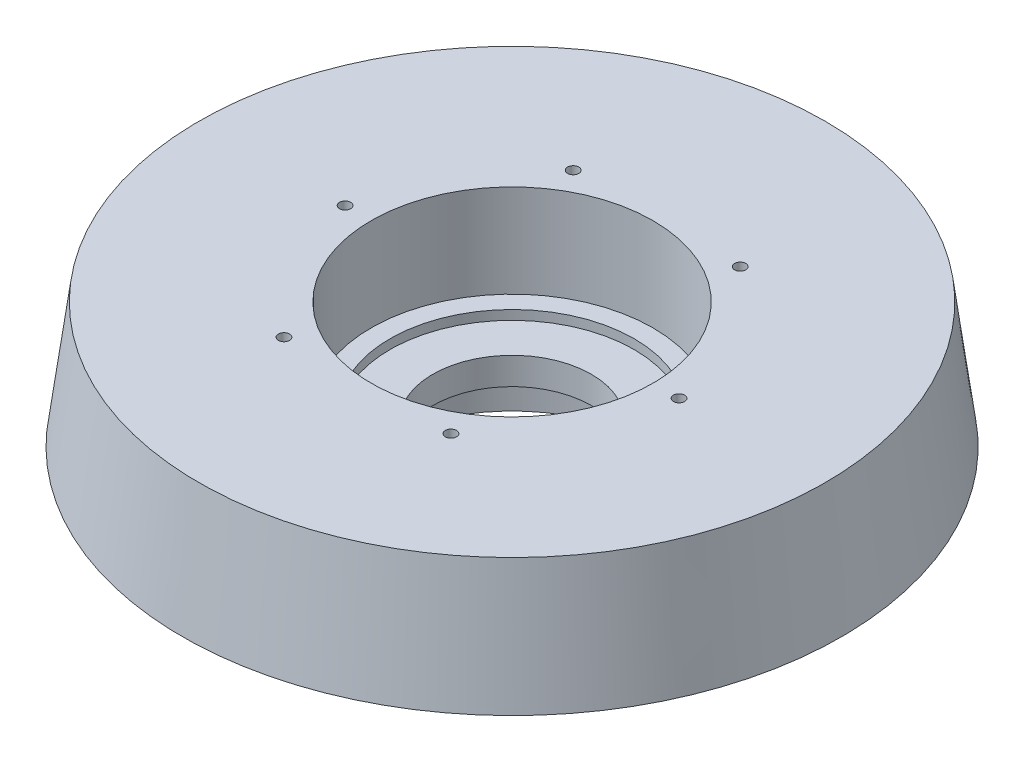
SolidWorks part; units mm, degrees
material "Plain Carbon Steel"
ref_plane "Front Plane" through (0, 0, 0) normal (0, 0, 1) x (1, 0, 0)
ref_plane "Top Plane" through (0, 0, 0) normal (0, 1, 0) x (1, 0, 0)
ref_plane "Right Plane" through (0, 0, 0) normal (1, 0, 0) x (0, 0, -1)
sketch "Sketch1" plane through (0, 0, 0) normal (0, 0, 1) x (1, 0, 0)
  line L0 (0, 0) -> (0, 317.4457) construction
  line L1 (-135, 0) -> (-135, 53)
  line L2 (-135, 53) -> (-117, 53)
  line L3 (-117, 53) -> (-117, 62)
  line L4 (-117, 62) -> (-76, 62)
  line L5 (-76, 62) -> (-76, 88)
  line L6 (-76, 88) -> (-117, 88)
  line L7 (-117, 88) -> (-117, 97)
  line L8 (-117, 97) -> (-135, 97)
  line L9 (-135, 97) -> (-135, 186)
  line L10 (-135, 186) -> (-300, 186)
  line L11 (-300, 186) -> (-315.7983, 66)
  line L12 (-315.7983, 66) -> (-185, 66)
  line L13 (-185, 66) -> (-185, 0)
  line L14 (-185, 0) -> (-135, 0)
  line L15 (0, 0) -> (-340.2912, 0) construction
  line L16 (-315.7983, 66) -> (-315.7983, 217.6526) construction
  dimension "D1" = 270
  dimension "D2" = 370
  dimension "D3" = 600
  dimension "D4" = 152
  dimension "D5" = 270
  dimension "D6" = 234
  dimension "D7" = 53
  dimension "D8" = 9
  dimension "D9" = 26
  dimension "D10" = 9
  dimension "D11" = 89
  dimension "D12" = 120
  dimension "D13" = 7.5
revolve "Revolve1" add sketch "Sketch1" angle 360 about L0
sketch "Sketch2" plane through (0, 186, 0) normal (0, 1, 0) x (1, 0, 0)
  line L0 (0, 0) -> (160, 0) construction
  circle A0 centre (0, 0) radius 160 construction
  dimension "D1" = 320
hole_wizard "1/2-13 Tapped Hole1" positions "3DSketch1" profile "Sketch3" tap size "1/2-13" standard "ANSI Inch"
sketch3d "3DSketch1"
  point P0 (160, 186, 0)
sketch "Sketch3" plane through (160, 186, 0) normal (1, 0, 0) x (0, 0, 1)
  line L0 (0, 0) -> (0, 28.6195)
  line L1 (0, 28.6195) -> (5.3581, 25.4)
  line L2 (5.3581, 25.4) -> (5.3581, 0)
  line L5 (5.3581, 0) -> (0, 0)
  line L10 (0, 28.6195) -> (-5.3581, 25.4) construction
  line L11 (0, -6.35) -> (0, 107.95) construction
  dimension "Tap Drill Dia." = 10.7163
  dimension "Tap Drill Depth" = 25.4
  dimension "Drill Angle" = 118
cosmetic thread "Hole Thread1" parameters "D1"=25.4, "D2"=12.7
pattern_circular "CirPattern1" count 6 over 360 about axis through (0, 0, 0) along (0, 1, 0) of "1/2-13 Tapped Hole1"
sketch "Sketch4" plane through (0, 0, 0) normal (0, -1, 0) x (1, 0, 0)
  line L0 (0, 0) -> (160, 0) construction
  circle A0 centre (0, 0) radius 160 construction
  dimension "D1" = 320
hole_wizard "1/2-13 Tapped Hole2" positions "3DSketch2" profile "Sketch5" tap size "1/2-13" standard "ANSI Inch"
sketch3d "3DSketch2"
  point P0 (160, 0, 0)
sketch "Sketch5" plane through (160, 0, 0) normal (1, 0, 0) x (0, 0, -1)
  line L0 (0, 0) -> (0, 34.4795)
  line L1 (0, 34.4795) -> (5.3581, 31.26)
  line L2 (5.3581, 31.26) -> (5.3581, 0)
  line L5 (5.3581, 0) -> (0, 0)
  line L10 (0, 34.4795) -> (-5.3581, 31.26) construction
  line L11 (0, -6.35) -> (0, 107.95) construction
  dimension "Tap Drill Dia." = 10.7163
  dimension "Tap Drill Depth" = 31.26
  dimension "Drill Angle" = 118
cosmetic thread "Hole Thread2" parameters "D1"=25.4, "D2"=12.7
pattern_circular "CirPattern2" count 6 over 360 about axis through (0, 0, 0) along (0, 1, 0) of "1/2-13 Tapped Hole2"
